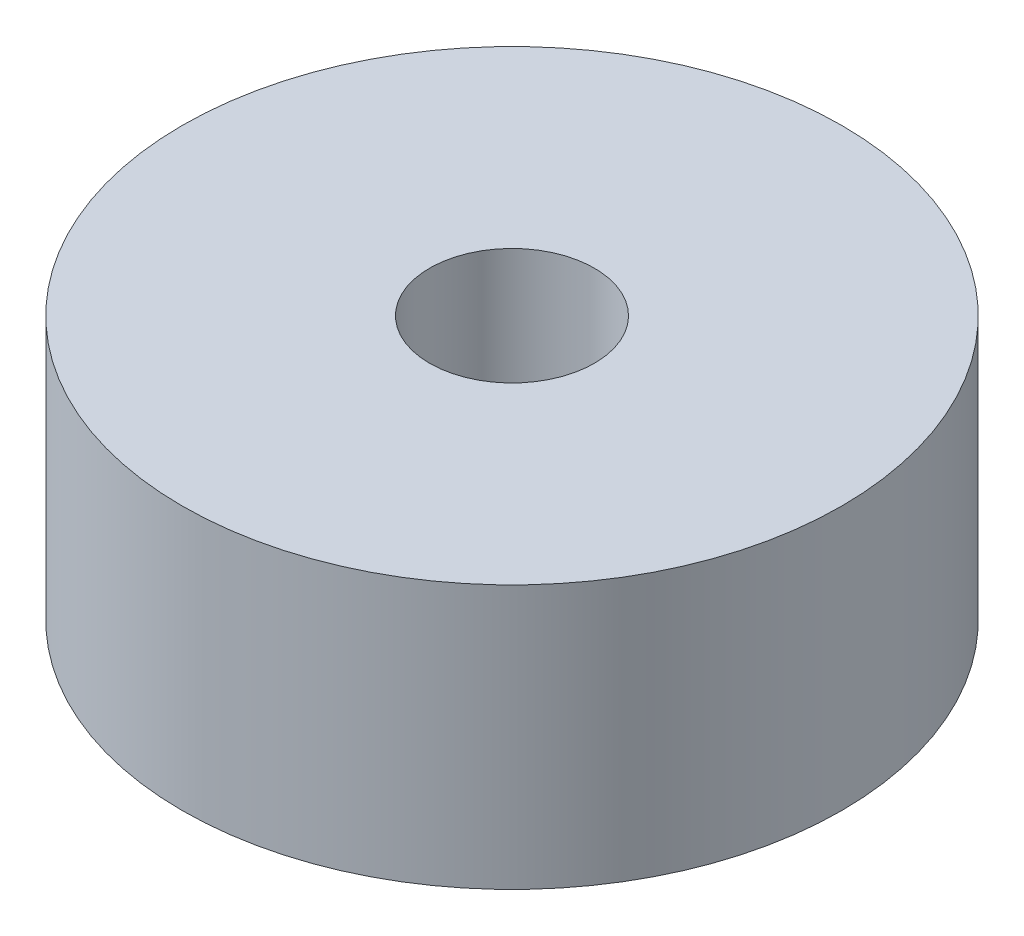
from build123d import *

# Parameters (mm, degrees)
SKETCH1_R           = 10
SKETCH1_R_2         = 2.5
BOSS_EXTRUDE1_DEPTH = 8


with BuildPart() as part:
    # Sketch1 → Boss-Extrude1 (new body)
    with BuildSketch(Plane(origin=(0, 0, 0), x_dir=(1, 0, 0), z_dir=(0, 1, 0))):
        with Locations(Location((0, 0, 0), (0, 0, 270))):
            Circle(SKETCH1_R)
        with Locations(Location((0, 0, 0), (0, 0, 270))):
            Circle(SKETCH1_R_2, mode=Mode.SUBTRACT)
    extrude(amount=BOSS_EXTRUDE1_DEPTH)


solid = part.part
